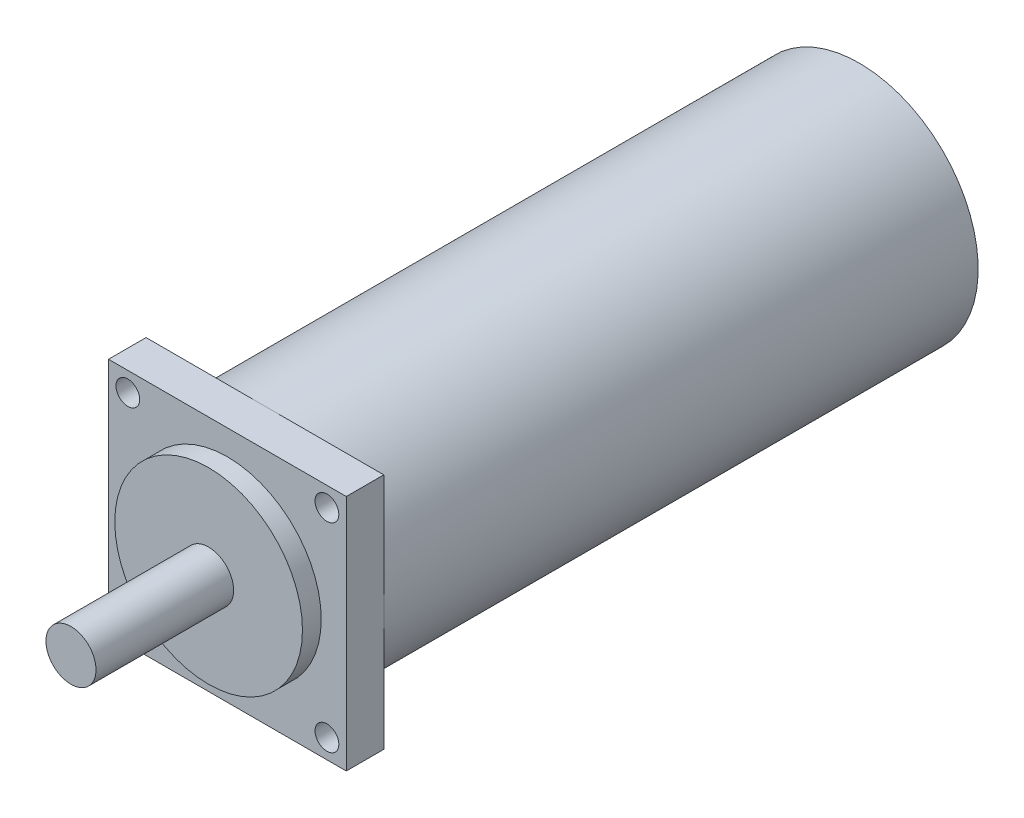
SolidWorks part; units mm, degrees
ref_plane "前视" through (0, 0, 0) normal (0, 0, 1) x (1, 0, 0)
ref_plane "上视" through (0, 0, 0) normal (0, 1, 0) x (1, 0, 0)
ref_plane "右视" through (0, 0, 0) normal (1, 0, 0) x (0, 0, -1)
sketch "草图1" plane through (0, 0, 0) normal (0, 0, 1) x (1, 0, 0)
  line L1 (0, 0) -> (38, 0)
  line L2 (0, 0) -> (0, 38)
  line L3 (0, 38) -> (38, 38)
  line L4 (38, 0) -> (38, 38)
  dimension "D1" = 38
  dimension "D2" = 38
extrude "拉伸1" add sketch "草图1" along normal blind 6
sketch "草图2" plane through (0, 0, 6) normal (0, 0, 1) x (1, 0, 0)
  line L0 (0, 19) -> (38, 19) construction
  line L1 (0, 38) -> (0, 0) construction
  line L2 (38, 0) -> (38, 38) construction
  circle A0 centre (19, 19) radius 15
  dimension "D1" = 30
extrude "拉伸2" add sketch "草图2" along normal blind 3
sketch "草图3" plane through (0, 0, 9) normal (0, 0, 1) x (1, 0, 0)
  circle A0 centre (19, 19) radius 4
  circle A1 centre (19, 19) radius 15 construction
  dimension "D1" = 8
extrude "拉伸3" add sketch "草图3" along normal blind 22
sketch "草图4" plane through (0, 0, 0) normal (0, 0, -1) x (-1, 0, 0)
  line L0 (-38, 19) -> (0, 19) construction
  line L1 (-38, 0) -> (-38, 38) construction
  line L2 (0, 38) -> (0, 0) construction
  circle A0 centre (-19, 19) radius 19
extrude "拉伸4" add sketch "草图4" along normal blind 97
sketch "草图5" plane through (0, 0, 6) normal (0, 0, 1) x (1, 0, 0)
  line L0 (19, 38) -> (19, 0) construction
  line L1 (0, 0) -> (38, 0) construction
  line L2 (0, 19) -> (38, 19) construction
  line L3 (0, 38) -> (0, 0) construction
  line L4 (38, 0) -> (38, 38) construction
  line L5 (3.0901, 34.9099) -> (19, 19) construction
  circle A0 centre (3.0901, 34.9099) radius 1.8987
  circle A1 centre (19, 19) radius 4 construction
  circle A2 centre (34.9099, 34.9099) radius 1.8987
  circle A3 centre (34.9099, 3.0901) radius 1.8987
  circle A4 centre (3.0901, 3.0901) radius 1.8987
  dimension "D1" = 22.5
  dimension "D2" = 45
extrude "切除-拉伸1" cut sketch "草图5" against normal up to next
chamfer "倒角1" distance 2 distance2 4 1 edges at (0, 19, -97)
